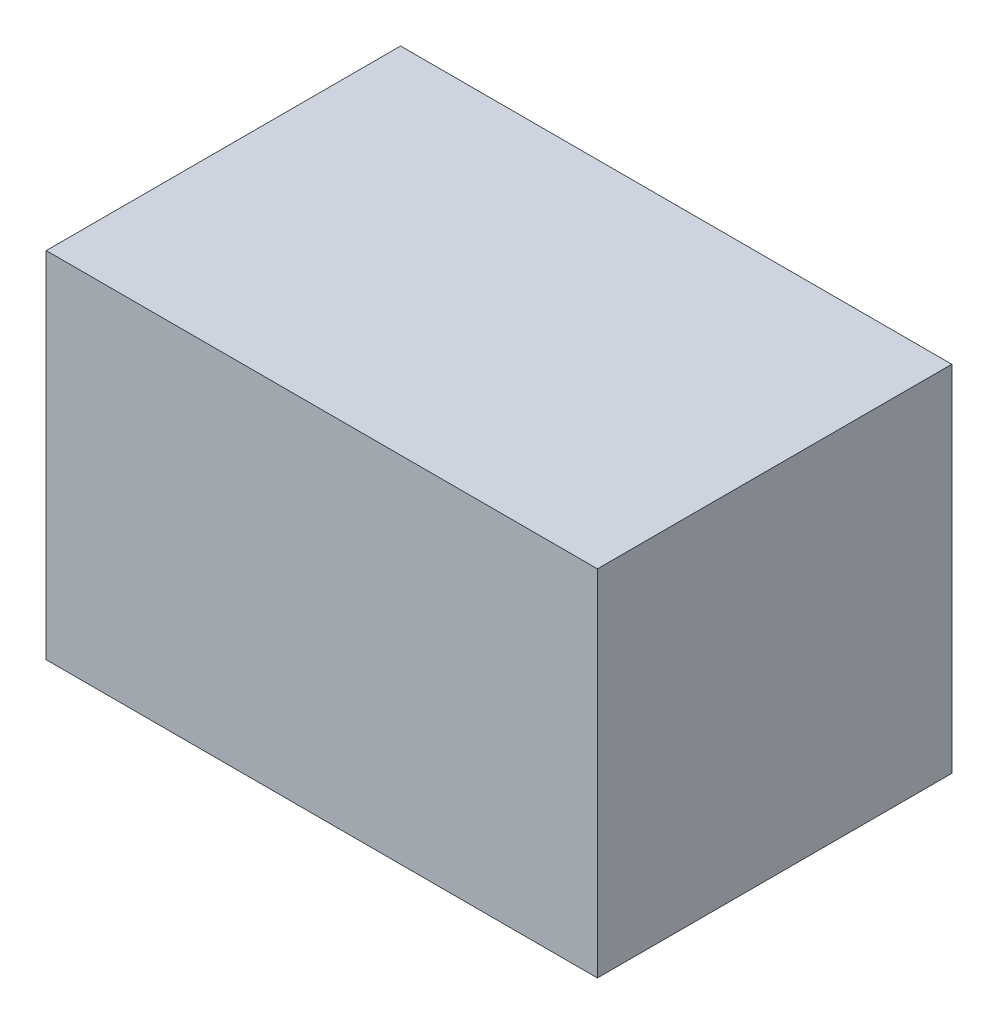
SolidWorks part; units mm, degrees
ref_plane "前视基准面" through (0, 0, 0) normal (0, 0, 1) x (1, 0, 0)
ref_plane "上视基准面" through (0, 0, 0) normal (0, 1, 0) x (1, 0, 0)
ref_plane "右视基准面" through (0, 0, 0) normal (1, 0, 0) x (0, 0, -1)
other "Configuration Table"
sketch "草图1" plane through (0, 0, 0) normal (0, 0, 1) x (1, 0, 0)
  line L0 (-70, -45) -> (70, -45)
  line L1 (70, -45) -> (70, 45)
  line L2 (70, 45) -> (-70, 45)
  line L3 (-70, 45) -> (-70, -45)
  point P0 (0, 0)
  dimension "D1" = 70
  dimension "D2" = 140
  dimension "D3" = 45
  dimension "D4" = 90
extrude "凸台-拉伸1" add sketch "草图1" against normal mid plane 90
